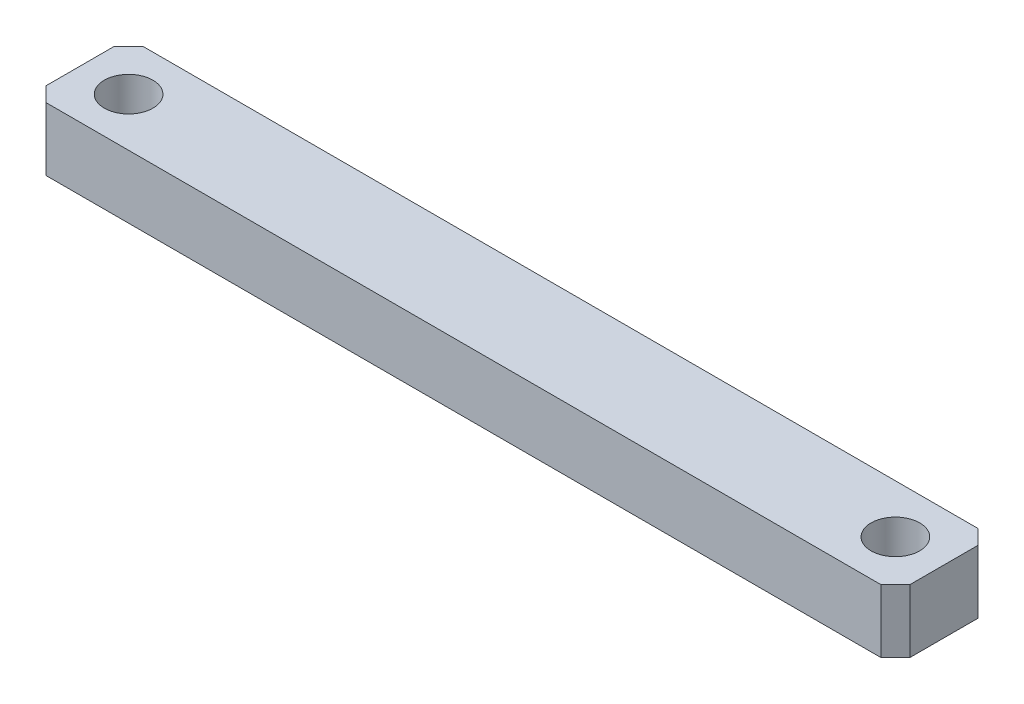
SolidWorks part; units mm, degrees
ref_plane "Front Plane" through (0, 0, 0) normal (0, 0, 1) x (1, 0, 0)
ref_plane "Top Plane" through (0, 0, 0) normal (0, 1, 0) x (1, 0, 0)
ref_plane "Right Plane" through (0, 0, 0) normal (1, 0, 0) x (0, 0, -1)
other "Configuration Table"
sketch "Sketch1" plane through (0, 0, 0) normal (0, 0, 1) x (1, 0, 0)
  line L1 (-88.9, 6.5) -> (88.9, 6.5)
  line L2 (-88.9, 6.5) -> (-88.9, -6.5)
  line L3 (-88.9, -6.5) -> (88.9, -6.5)
  line L4 (88.9, 6.5) -> (88.9, -6.5)
  line L5 (-88.9, 6.5) -> (88.9, -6.5) construction
  line L6 (-88.9, -6.5) -> (88.9, 6.5) construction
  point P0 (0, 0)
  dimension "D1" = 177.8
  dimension "D2" = 13
extrude "Boss-Extrude1" add sketch "Sketch1" along normal blind 20
chamfer "Chamfer1" distance 3 angle 45 4 edges at (88.9, 0, 0) (-88.9, 0, 0) (-88.9, 0, 20) (88.9, 0, 20)
sketch "Sketch2" plane through (0, 6.5, 0) normal (0, 1, 0) x (1, 0, 0)
  line L0 (85.9, 0) -> (-85.9, 0) construction
  line L1 (-88.9, -17) -> (-88.9, -3) construction
  circle A0 centre (-78.9, -10) radius 5
  dimension "D3" = 10
  dimension "D1" = 10
  dimension "D2" = 10
extrude "Cut-Extrude1" cut sketch "Sketch2" against normal blind 13
pattern_linear "LPattern1" count 2 spacing 157.8 along (1, 0, 0) of "Cut-Extrude1"
